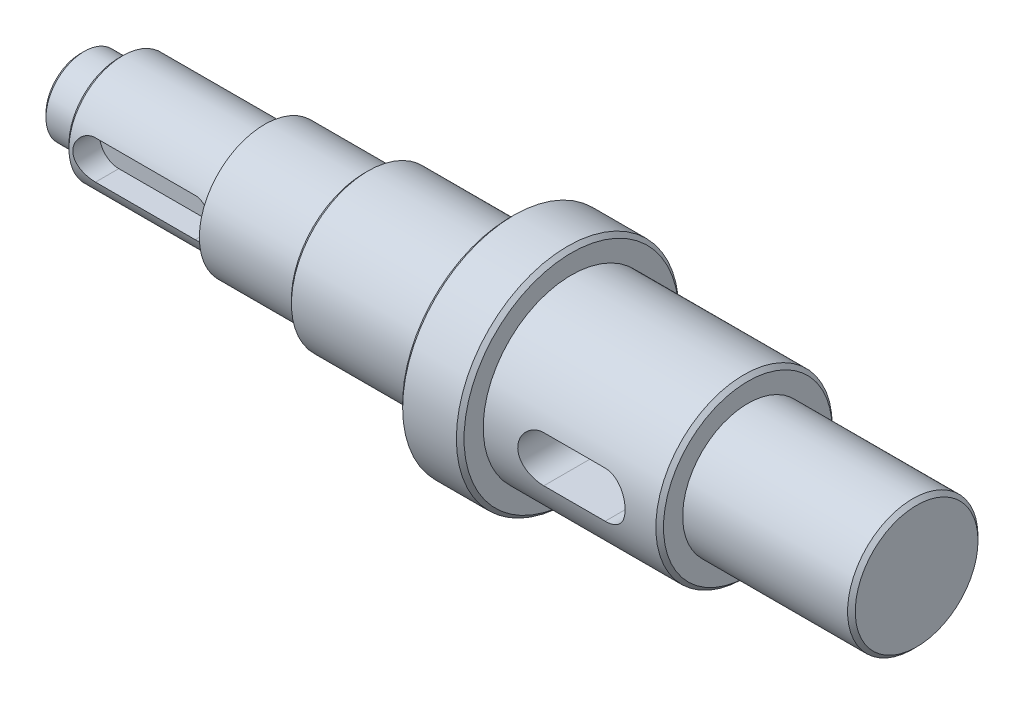
from build123d import *

# Parameters (mm, degrees)
SKETCH1_R           = 5
BOSS_EXTRUDE1_DEPTH = 5
SKETCH2_R           = 7
BOSS_EXTRUDE2_DEPTH = 19
SKETCH3_R           = 8.5
BOSS_EXTRUDE3_DEPTH = 13
SKETCH4_R           = 10
BOSS_EXTRUDE4_DEPTH = 19
SKETCH5_R           = 14.5
BOSS_EXTRUDE5_DEPTH = 8
SKETCH6_R           = 11.5
BOSS_EXTRUDE6_DEPTH = 23
SKETCH7_R           = 8.5
BOSS_EXTRUDE7_DEPTH = 22
CHAMFER1_SIZE       = 0.5
CUT_EXTRUDE2_START  = 7
CUT_EXTRUDE2_DEPTH  = 3.5
CUT_EXTRUDE3_START  = 11.5
CUT_EXTRUDE3_DEPTH  = 6.5
FILLET1_R           = 2


with BuildPart() as part:
    # Sketch1 → Boss-Extrude1 (new body)
    with BuildSketch(Plane(origin=(0, 0, 0), x_dir=(0, 0, -1), z_dir=(1, 0, 0))):
        Circle(SKETCH1_R)
    extrude(amount=BOSS_EXTRUDE1_DEPTH)

    # Sketch2 → Boss-Extrude2 (add)
    with BuildSketch(Plane(origin=(5, 0, 0), x_dir=(0, 0, -1), z_dir=(1, 0, 0))):
        Circle(SKETCH2_R)
    extrude(amount=BOSS_EXTRUDE2_DEPTH)

    # Sketch3 → Boss-Extrude3 (add)
    with BuildSketch(Plane(origin=(24, 0, 0), x_dir=(0, 0, -1), z_dir=(1, 0, 0))):
        with Locations(Location((0, 0, 0), (0, 0, 180))):
            Circle(SKETCH3_R)
    extrude(amount=BOSS_EXTRUDE3_DEPTH)

    # Sketch4 → Boss-Extrude4 (add)
    with BuildSketch(Plane(origin=(37, 0, 0), x_dir=(0, 0, -1), z_dir=(1, 0, 0))):
        Circle(SKETCH4_R)
    extrude(amount=BOSS_EXTRUDE4_DEPTH)

    # Sketch5 → Boss-Extrude5 (add)
    with BuildSketch(Plane(origin=(56, 0, 0), x_dir=(0, 0, -1), z_dir=(1, 0, 0))):
        Circle(SKETCH5_R)
    extrude(amount=BOSS_EXTRUDE5_DEPTH)

    # Sketch6 → Boss-Extrude6 (add)
    with BuildSketch(Plane(origin=(64, 0, 0), x_dir=(0, 0, -1), z_dir=(1, 0, 0))):
        Circle(SKETCH6_R)
    extrude(amount=BOSS_EXTRUDE6_DEPTH)

    # Sketch7 → Boss-Extrude7 (add)
    with BuildSketch(Plane(origin=(87, 0, 0), x_dir=(0, 0, -1), z_dir=(1, 0, 0))):
        with Locations(Location((0, 0, 0), (0, 0, 180))):
            Circle(SKETCH7_R)
    extrude(amount=BOSS_EXTRUDE7_DEPTH)

    # Chamfer1
    chamfer1_edges = [part.edges().sort_by_distance(p)[0] for p in [
        (37, 0, 10),
        (56, 0, 14.5),
        (0, 0, 5),
        (64, 0, 14.5),
        (87, 0, 11.5),
        (109, 0, -8.5),
        (5, 0, 7),
    ]]
    chamfer(chamfer1_edges, length=CHAMFER1_SIZE)

    # Sketch8 → Cut-Extrude2 (cut)
    with BuildSketch(Plane.XY.offset(CUT_EXTRUDE2_START)):
        with BuildLine():
            Line((8.5, 2.5), (21.5, 2.5))
            ThreePointArc((21.5, 2.5), (24, 0), (21.5, -2.5))
            Line((21.5, -2.5), (8.5, -2.5))
            ThreePointArc((8.5, -2.5), (6, 0), (8.5, 2.5))
        make_face()
    extrude(amount=-CUT_EXTRUDE2_DEPTH, mode=Mode.SUBTRACT)

    # Sketch9 → Cut-Extrude3 (cut)
    with BuildSketch(Plane.XY.offset(CUT_EXTRUDE3_START)):
        with BuildLine():
            Line((71.5, 3), (79.5, 3))
            ThreePointArc((79.5, 3), (82.5, 0), (79.5, -3))
            Line((79.5, -3), (71.5, -3))
            ThreePointArc((71.5, -3), (68.5, 0), (71.5, 3))
        make_face()
    extrude(amount=-CUT_EXTRUDE3_DEPTH, mode=Mode.SUBTRACT)

    # Fillet1
    fillet1_edges = [part.edges().sort_by_distance(p)[0] for p in [
        (56, 0, 10),
    ]]
    fillet(fillet1_edges, radius=FILLET1_R)


solid = part.part
